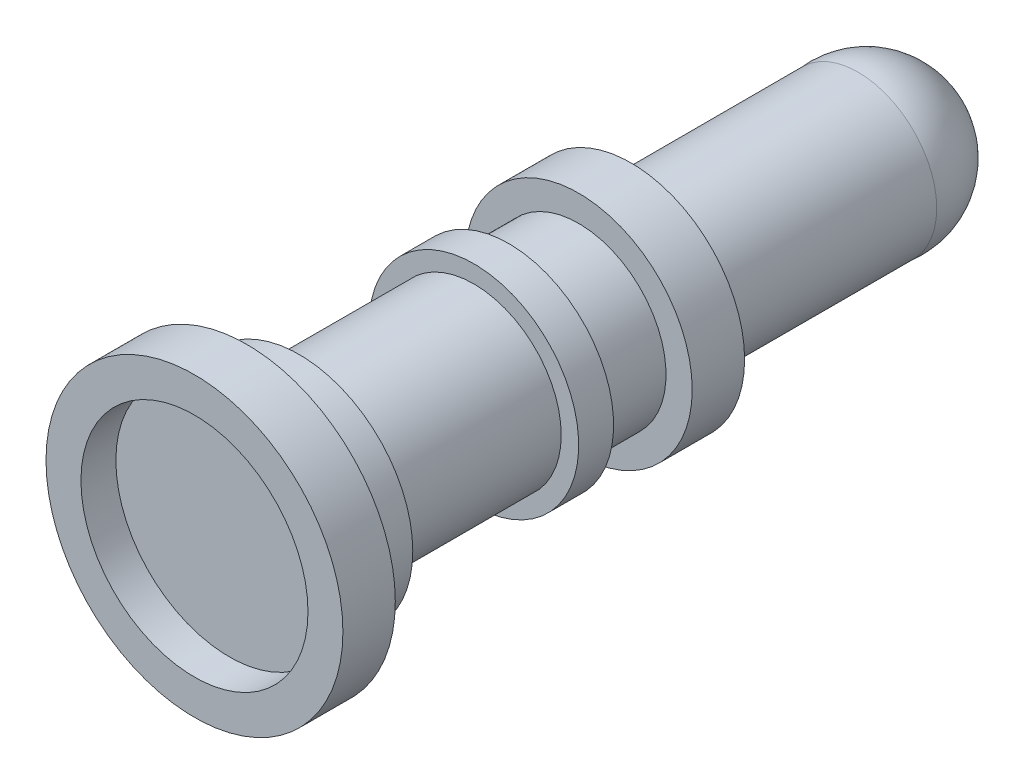
from build123d import *

# Parameters (mm, degrees)
SKETCH1_R                = 5
BOSS_EXTRUDE1_DEPTH      = 3
SKETCH2_R                = 6.5
BOSS_EXTRUDE2_DEPTH      = 4
BOSS_EXTRUDE3_DEPTH      = 2
BOSS_EXTRUDE3_DEPTH_BACK = 1
SKETCH3_R                = 8.5
SKETCH3_R_2              = 6.5
SKETCH4_R                = 5
BOSS_EXTRUDE4_DEPTH      = 9
SKETCH5_R                = 6
BOSS_EXTRUDE5_DEPTH      = 2
SKETCH7_R                = 5
BOSS_EXTRUDE6_DEPTH      = 4
BOSS_EXTRUDE7_START      = 3
SKETCH8_R                = 6.5
BOSS_EXTRUDE7_DEPTH      = 3
SKETCH10_R               = 4.5
BOSS_EXTRUDE8_DEPTH      = 13
DOME1_FACE_RADIUS        = 4.5
DOME1_HEIGHT             = 5
SKETCH11_R               = 1
CUT_EXTRUDE1_DEPTH       = 26


with BuildPart() as part:
    # Sketch1 → Boss-Extrude1 (new body)
    with BuildSketch(Plane.XY):
        with Locations((3, 0)):
            Circle(SKETCH1_R)
    extrude(amount=-BOSS_EXTRUDE1_DEPTH)

    # Sketch2 → Boss-Extrude2 (add)
    with BuildSketch(Plane.XY):
        with Locations((3, 0)):
            Circle(SKETCH2_R)
    extrude(amount=BOSS_EXTRUDE2_DEPTH)

    # Sketch3 → Boss-Extrude3 (add, two sides: drawn at the far end of the back side and taken through both)
    with BuildSketch(Plane.XY.offset(4).offset(-BOSS_EXTRUDE3_DEPTH_BACK)):
        with Locations((3, 0)):
            Circle(SKETCH3_R)
        with Locations((3, 0)):
            Circle(SKETCH3_R_2, mode=Mode.SUBTRACT)
    extrude(amount=BOSS_EXTRUDE3_DEPTH + BOSS_EXTRUDE3_DEPTH_BACK)

    # Sketch4 → Boss-Extrude4 (add)
    with BuildSketch(Plane(origin=(0, 0, -3), x_dir=(-1, 0, 0), z_dir=(0, 0, -1))):
        with Locations(Location((-3, 0, 0), (0, 0, 180))):
            Circle(SKETCH4_R)
    extrude(amount=BOSS_EXTRUDE4_DEPTH)

    # Sketch5 → Boss-Extrude5 (add)
    with BuildSketch(Plane(origin=(0, 0, -12), x_dir=(-1, 0, 0), z_dir=(0, 0, -1))):
        with Locations((-3, 0)):
            Circle(SKETCH5_R)
    extrude(amount=-BOSS_EXTRUDE5_DEPTH)

    # Sketch7 → Boss-Extrude6 (add)
    with BuildSketch(Plane(origin=(0, 0, -12), x_dir=(-1, 0, 0), z_dir=(0, 0, -1))):
        with Locations(Location((-3, 0, 0), (0, 0, 180))):
            Circle(SKETCH7_R)
    extrude(amount=BOSS_EXTRUDE6_DEPTH)

    # Sketch8 → Boss-Extrude7 (add)
    with BuildSketch(Plane(origin=(0, 0, -16), x_dir=(-1, 0, 0), z_dir=(0, 0, -1)).offset(BOSS_EXTRUDE7_START)):
        with Locations(Location((-3, 0, 0), (0, 0, 180))):
            Circle(SKETCH8_R)
    extrude(amount=-BOSS_EXTRUDE7_DEPTH)

    # Sketch10 → Boss-Extrude8 (add)
    with BuildSketch(Plane(origin=(0, 0, -19), x_dir=(-1, 0, 0), z_dir=(0, 0, -1))):
        with Locations((-3, 0)):
            Circle(SKETCH10_R)
    extrude(amount=BOSS_EXTRUDE8_DEPTH)

    # Dome1: a dome of height H over a round flat face of radius A is a cap of a sphere of radius (A * A + H * H) / (2 * H)
    dome1_r = (DOME1_FACE_RADIUS * DOME1_FACE_RADIUS + DOME1_HEIGHT * DOME1_HEIGHT) / (2 * DOME1_HEIGHT)
    dome1_base = Plane((3, 0, -32), z_dir=(0, 0, -1))
    with Locations(dome1_base.offset(DOME1_HEIGHT - dome1_r)):
        dome1_ball = Sphere(dome1_r, mode=Mode.PRIVATE)
    add(split(dome1_ball, bisect_by=dome1_base, keep=Keep.TOP, mode=Mode.PRIVATE))

    # Sketch11 → Cut-Extrude1 (cut)
    with BuildSketch(Plane(origin=(0, 0, -19), x_dir=(-1, 0, 0), z_dir=(0, 0, -1))):
        with Locations(Location((-3, 0, 0), (0, 0, 180))):
            Circle(SKETCH11_R)
    extrude(amount=CUT_EXTRUDE1_DEPTH, mode=Mode.SUBTRACT)


solid = part.part
